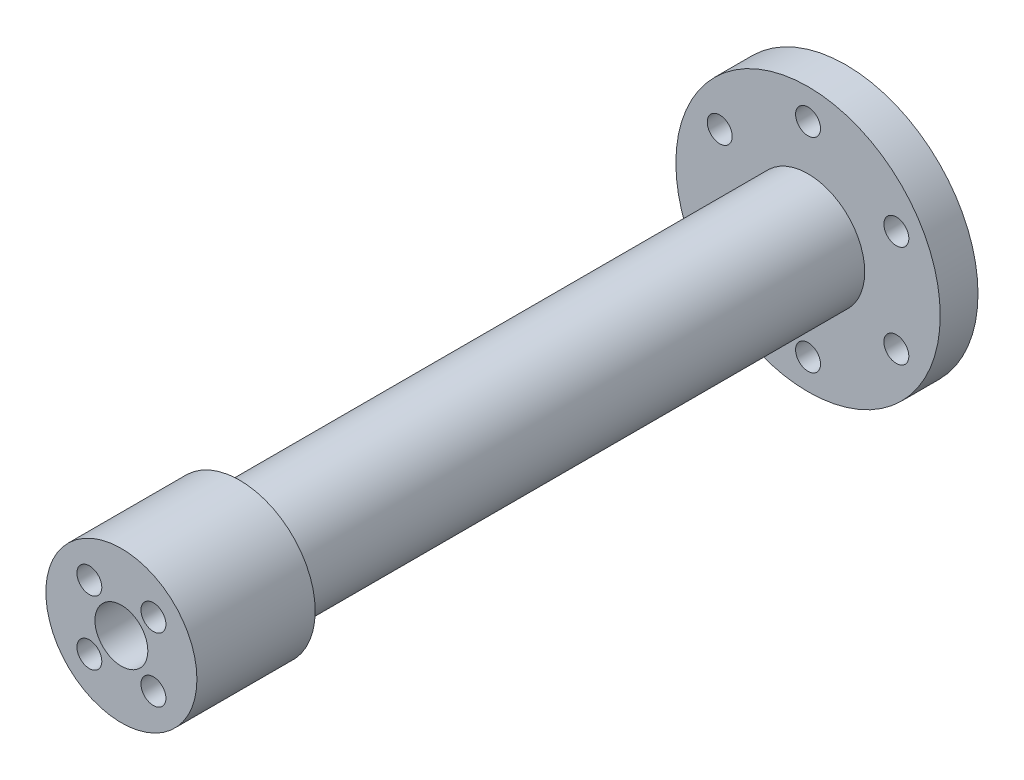
from build123d import *

# Parameters (mm, degrees)
SKETCH_1_R          = 17.5
EXTRUDE_1_DEPTH     = 5
SKETCH_2_R          = 7.5
EXTRUDE_2_DEPTH     = 90.91
SKETCH_3_R          = 1.65
SKETCH_3_R_2        = 3.5
CUT_EXTRUDE_1_DEPTH = 1000
SKETCH_4_R          = 10
SKETCH_4_R_2        = 4
EXTRUDE_3_DEPTH     = 15.66
SKETCH_5_R          = 1.65
CUT_EXTRUDE_2_DEPTH = 8


with BuildPart() as part:
    # 草图1 → 凸台-拉伸1 (new body)
    with BuildSketch(Plane.XY):
        Circle(SKETCH_1_R)
    extrude(amount=EXTRUDE_1_DEPTH)

    # 草图2 → 凸台-拉伸2 (add)
    with BuildSketch(Plane.XY.offset(5)):
        Circle(SKETCH_2_R)
    extrude(amount=EXTRUDE_2_DEPTH)

    # 草图3 → 切除-拉伸1 (cut)
    with BuildSketch(Plane(origin=(0, 0, 0), x_dir=(-1, 0, 0), z_dir=(0, 0, -1))):
        with Locations((0, 13.5)):
            Circle(SKETCH_3_R)
        with Locations((11.691342951, 6.75)):
            Circle(SKETCH_3_R)
        with Locations((11.691342951, -6.75)):
            Circle(SKETCH_3_R)
        with Locations((0, -13.5)):
            Circle(SKETCH_3_R)
        with Locations((-11.691342951, -6.75)):
            Circle(SKETCH_3_R)
        with Locations((-11.691342951, 6.75)):
            Circle(SKETCH_3_R)
        Circle(SKETCH_3_R_2)
    extrude(amount=-CUT_EXTRUDE_1_DEPTH, mode=Mode.SUBTRACT)

    # 草图4 → 凸台-拉伸3 (add)
    with BuildSketch(Plane.XY.offset(95.91)):
        Circle(SKETCH_4_R)
        Circle(SKETCH_4_R_2, mode=Mode.SUBTRACT)
    extrude(amount=-EXTRUDE_3_DEPTH)

    # 草图5 → 切除-拉伸2 (cut)
    with BuildSketch(Plane.XY.offset(95.91)):
        with Locations((-4.242640687, 4.242640687)):
            Circle(SKETCH_5_R)
        with Locations((-4.242640687, -4.242640687)):
            Circle(SKETCH_5_R)
        with Locations((4.242640687, -4.242640687)):
            Circle(SKETCH_5_R)
        with Locations((4.242640687, 4.242640687)):
            Circle(SKETCH_5_R)
    extrude(amount=-CUT_EXTRUDE_2_DEPTH, mode=Mode.SUBTRACT)


solid = part.part
